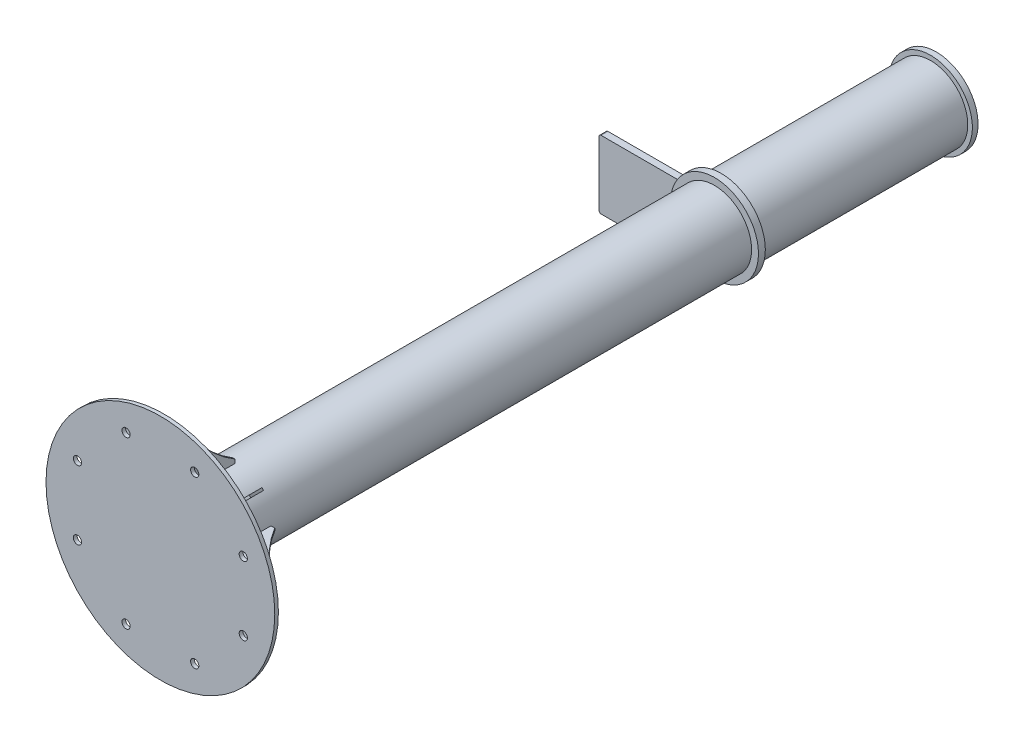
SolidWorks part; units mm, degrees
ref_plane "Front Plane" through (0, 0, 0) normal (0, 0, 1) x (1, 0, 0)
ref_plane "Top Plane" through (0, 0, 0) normal (0, 1, 0) x (1, 0, 0)
ref_plane "Right Plane" through (0, 0, 0) normal (1, 0, 0) x (0, 0, -1)
other "Configuration Table"
sketch "Sketch1" plane through (0, 0, 0) normal (0, 0, 1) x (1, 0, 0)
  circle A0 centre (0, 0) radius 162.5
  circle A1 centre (0, 0) radius 142.5
  dimension "D1" = 325
  dimension "D2" = 285
extrude "Boss-Extrude1" add sketch "Sketch1" along normal blind 3363.5
sketch "Sketch2" plane through (0, 0, 3363.5) normal (0, 0, 1) x (1, 0, 0)
  circle A0 centre (0, 0) radius 162.5
  circle A1 centre (0, 0) radius 192.5
  dimension "D1" = 385
extrude "Boss-Extrude2" add sketch "Sketch2" against normal blind 30 from offset 2406 offset against normal yes
sketch "Sketch3" plane through (0, 0, 3363.5) normal (0, 0, 1) x (1, 0, 0)
  circle A0 centre (0, 0) radius 500
  dimension "D1" = 1000
extrude "Boss-Extrude3" add sketch "Sketch3" along normal blind 16
sketch "Sketch4" plane through (0, 0, 0) normal (1, 0, 0) x (0, 0, -1)
  line L0 (-3058.5, 150.1038) -> (-3058.5, 179.1591)
  line L1 (-3255.0575, 377.5) -> (-3363.5, 377.5)
  line L2 (-3363.5, -500) -> (-3363.5, 500) construction
  line L3 (-3363.5, 377.5) -> (-3363.5, 150.1038)
  line L4 (-3363.5, -162.5) -> (-3363.5, 162.5) construction
  line L5 (-3363.5, 150.1038) -> (-3058.5, 150.1038)
  line L6 (-957.5, 162.5) -> (-3363.5, 162.5) construction
  arc A0 (-3058.5, 179.1591) -> (-3255.0575, 377.5) centre (-2766.3346, 665.2628) cw
  dimension "D1" = 305
  dimension "D2" = 215
extrude "Boss-Extrude4" add sketch "Sketch4" along normal mid plane 10
pattern_circular "CirPattern1" count 8 over 360 about axis through (0, 0, 0) along (0, 0, 1) of "Boss-Extrude4"
sketch "Sketch5" plane through (0, 0, 3363.5) normal (0, 0, -1) x (-1, 0, 0)
  line L0 (0, 0) -> (0, 392.3468) construction
  line L1 (0, 0) -> (150.1446, 362.4811) construction
  circle A0 centre (0, 0) radius 392.3468 construction
  circle A1 centre (150.1446, 362.4811) radius 18
  circle A2 centre (362.4811, 150.1446) radius 18
  circle A3 centre (362.4811, -150.1446) radius 18
  circle A4 centre (150.1446, -362.4811) radius 18
  circle A5 centre (-150.1446, -362.4811) radius 18
  circle A6 centre (-362.4811, -150.1446) radius 18
  circle A7 centre (-362.4811, 150.1446) radius 18
  circle A8 centre (-150.1446, 362.4811) radius 18
  point P22 (0, 0)
  dimension "D2" = 36
  dimension "D1" = 22.5
  dimension "D3" = 8
extrude "Cut-Extrude1" cut sketch "Sketch5" against normal through all
sketch "Sketch6" plane through (0, 0, 0) normal (0, 0, -1) x (-1, 0, 0)
  circle A0 centre (0, 0) radius 182.5
  dimension "D1" = 365
extrude "Boss-Extrude5" add sketch "Sketch6" along normal mid plane 25
sketch "Sketch7" plane through (0, 0, -12.5) normal (0, 0, -1) x (-1, 0, 0)
  line L0 (129.7122, 59) -> (540, 59)
  line L1 (550, 49) -> (550, 0)
  line L2 (550, 0) -> (550, -229)
  line L3 (540, -239) -> (267.2588, -239)
  line L4 (0, 0) -> (747.4649, 0) construction
  line L5 (257.2588, -229) -> (257.2588, -99)
  line L6 (217.2588, -59) -> (129.7122, -59)
  circle A0 centre (0, 0) radius 182.5 construction
  arc A1 (129.7122, -59) -> (129.7122, 59) centre (0, 0) ccw
  arc A2 (257.2588, -99) -> (217.2588, -59) centre (217.2588, -99) ccw
  arc A3 (267.2588, -239) -> (257.2588, -229) centre (267.2588, -229) cw
  arc A4 (550, 49) -> (540, 59) centre (540, 49) ccw
  arc A5 (550, -229) -> (540, -239) centre (540, -229) cw
  dimension "D2" = 285
  dimension "D3" = 40
  dimension "D4" = 10
  dimension "D1" = 550
  dimension "D5" = 59
  dimension "D6" = 59
  dimension "D7" = 180
extrude "Boss-Extrude6" add sketch "Sketch7" against normal blind 30 from offset 895
